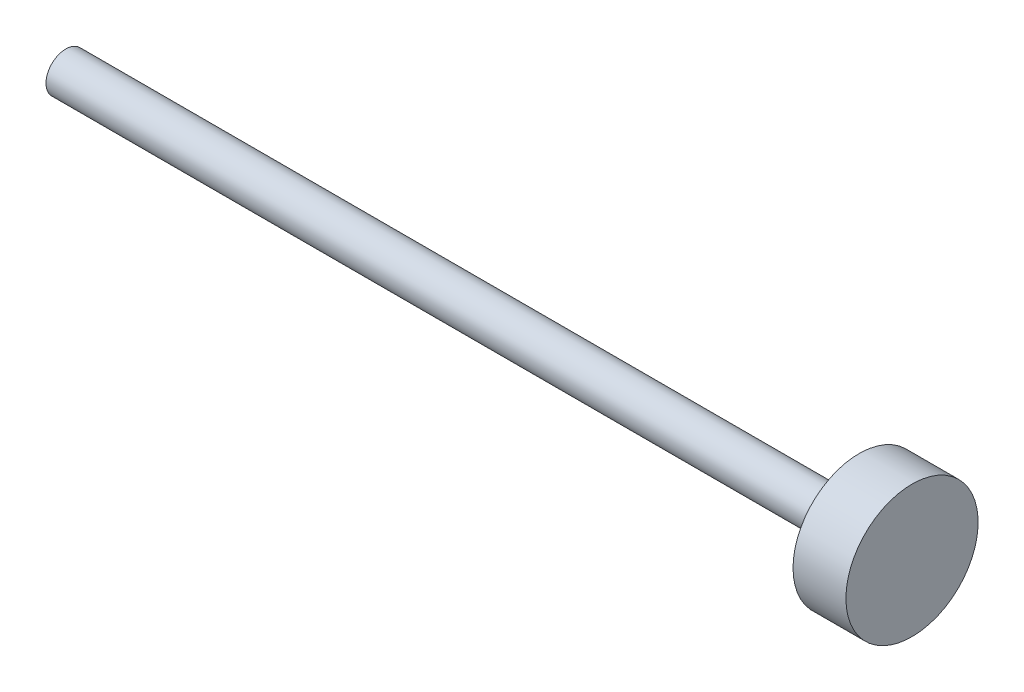
from build123d import *


with BuildPart() as part:
    # Sketch1 → Revolve1 (revolve)
    with BuildSketch(Plane.XY, mode=Mode.PRIVATE) as revolve1_sk:
        Polygon((214.220434241, 242.08300471), (534.220434241, 242.08300471), (534.220434241, 267.08300471), (514.220434241, 267.08300471), (514.220434241, 249.58300471), (214.220434241, 249.58300471), align=None)
    revolve(revolve1_sk.sketch.rotate(Axis((214.220434241, 242.08300471, 0), (1, 0, 0)), 90), axis=Axis((214.220434241, 242.08300471, 0), (1, 0, 0)))


solid = part.part
